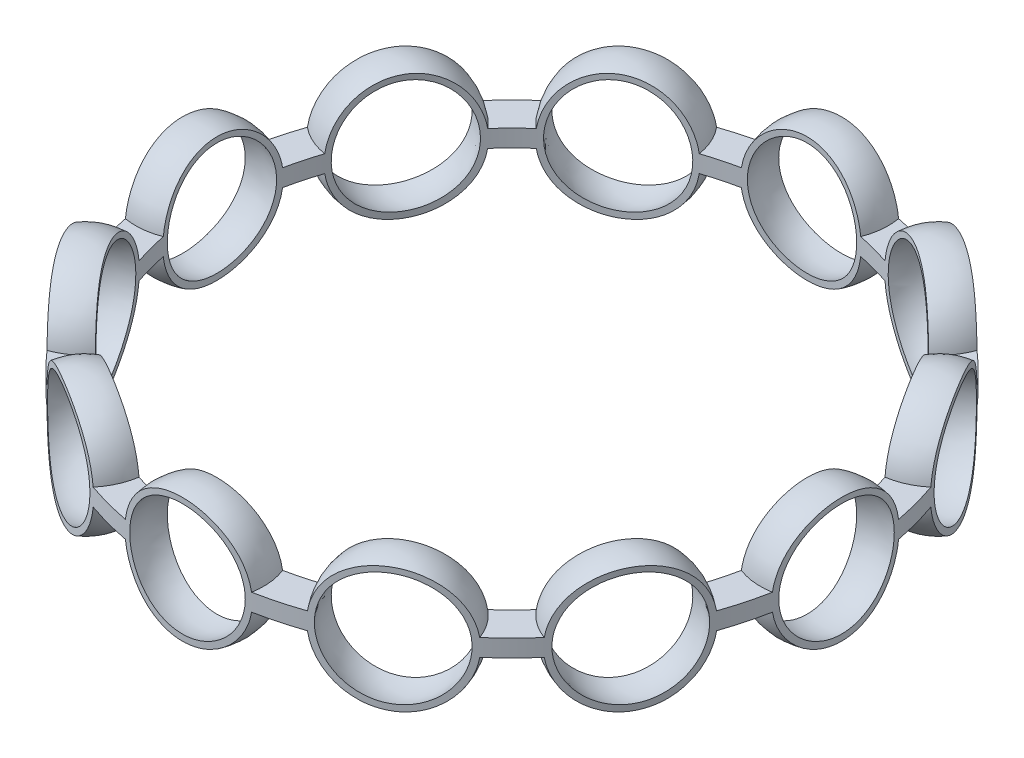
SolidWorks part; units mm, degrees
ref_plane "Front Plane" through (0, 0, 0) normal (0, 0, 1) x (1, 0, 0)
ref_plane "Top Plane" through (0, 0, 0) normal (0, 1, 0) x (1, 0, 0)
ref_plane "Right Plane" through (0, 0, 0) normal (1, 0, 0) x (0, 0, -1)
other "Configuration Table"
sketch "Sketch1" plane through (0, 0, 0) normal (0, 1, 0) x (1, 0, 0)
  circle A0 centre (0, 0) radius 50
  dimension "D1" = 100
extrude "Boss-Extrude1" add sketch "Sketch1" along normal mid plane 2
sketch "Sketch2" plane through (0, 0, 0) normal (1, 0, 0) x (0, 0, -1)
  line L0 (36.25, 22.3209) -> (36.25, -21.1866) construction
  line L1 (36.25, 7.5) -> (36.25, -7.5)
  arc A0 (36.25, -7.5) -> (36.25, 7.5) centre (36.25, 0) ccw
  dimension "D2" = 15
  dimension "D1" = 36.25
revolve "Revolve1" add sketch "Sketch2" angle 360 about L0
pattern_circular "CirPattern1" count 12 over 360 about axis through (0, 0, 0) along (0, 1, 0) of "Revolve1"
sketch "Sketch3" plane through (0, 0, 0) normal (0, 1, 0) x (1, 0, 0)
  circle A0 centre (0, 0) radius 36.25 construction
  circle A1 centre (0, 0) radius 38.25
  circle A2 centre (0, 0) radius 34.25
  dimension "D1" = 72.5
  dimension "D2" = 2
  dimension "D3" = 2
extrude "Cut-Extrude2" cut sketch "Sketch3" against normal through all and the other way through all flip side to cut
sketch "Sketch4" plane through (0, 0, 0) normal (1, 0, 0) x (0, 0, -1)
  line L0 (0, 0) -> (56.2722, 0) construction
  line L1 (36.25, 18.0894) -> (36.25, -17.9988) construction
  line L2 (36.25, 6.8953) -> (36.25, -6.8047)
  arc A0 (36.25, -6.8047) -> (36.25, 6.8953) centre (36.25, 0.0453) ccw
  dimension "D2" = 13.7
  dimension "D1" = 36.25
revolve "Cut-Revolve1" cut sketch "Sketch4" angle 360 about L1
pattern_circular "CirPattern2" count 12 over 360 about axis through (0, 0, 0) along (0, 1, 0) of "Cut-Revolve1"
